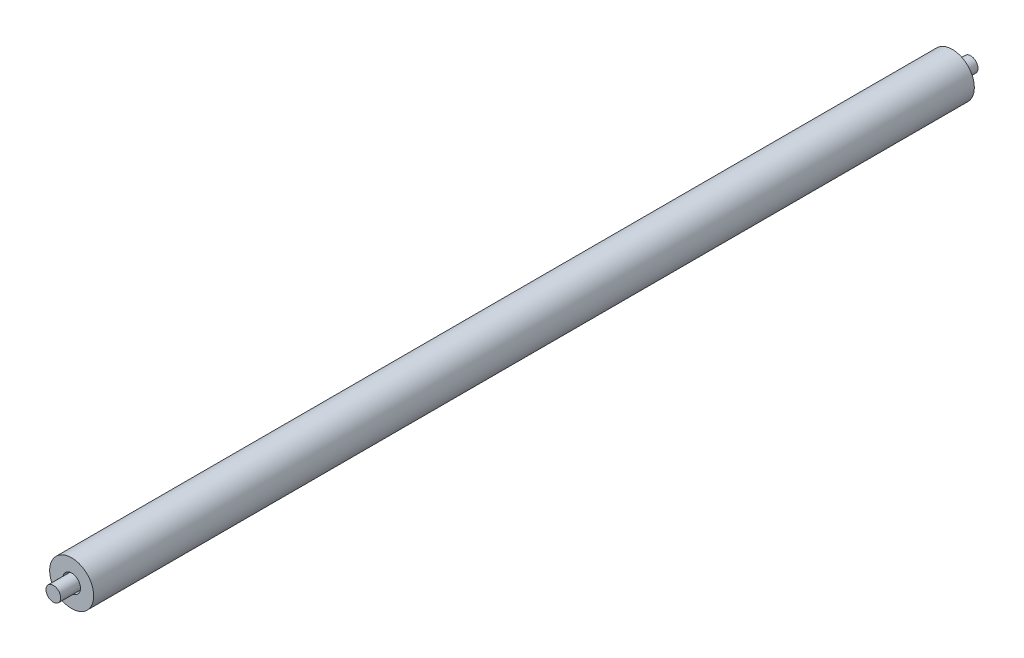
SolidWorks part; units mm, degrees
ref_plane "前视基准面" through (0, 0, 0) normal (0, 0, 1) x (1, 0, 0)
ref_plane "上视基准面" through (0, 0, 0) normal (0, 1, 0) x (1, 0, 0)
ref_plane "右视基准面" through (0, 0, 0) normal (1, 0, 0) x (0, 0, -1)
other "Configuration Table"
sketch "草图1" plane through (0, 0, 0) normal (0, 0, 1) x (1, 0, 0)
  circle A0 centre (0, 0) radius 10
  dimension "D1" = 20
extrude "凸台-拉伸1" add sketch "草图1" along normal mid plane 1250
sketch "草图2" plane through (0, 0, 0) normal (0, 0, 1) x (1, 0, 0)
  circle A0 centre (0, 0) radius 10 construction
  circle A1 centre (0, 0) radius 10
  circle A2 centre (0, 0) radius 30
  dimension "D1" = 60
extrude "凸台-拉伸2" add sketch "草图2" along normal mid plane 1200 separate body
sketch "草图3" plane through (0, 0, 600) normal (0, 0, 1) x (1, 0, 0)
  circle A0 centre (0, 0) radius 5
  circle A1 centre (0, 0) radius 12
  dimension "D1" = 24
  dimension "D2" = 10
extrude "切除-拉伸1" cut sketch "草图3" against normal blind 10
mirror "镜向1" about plane through (0, 0, 0) normal (0, 0, 1) of "切除-拉伸1"
